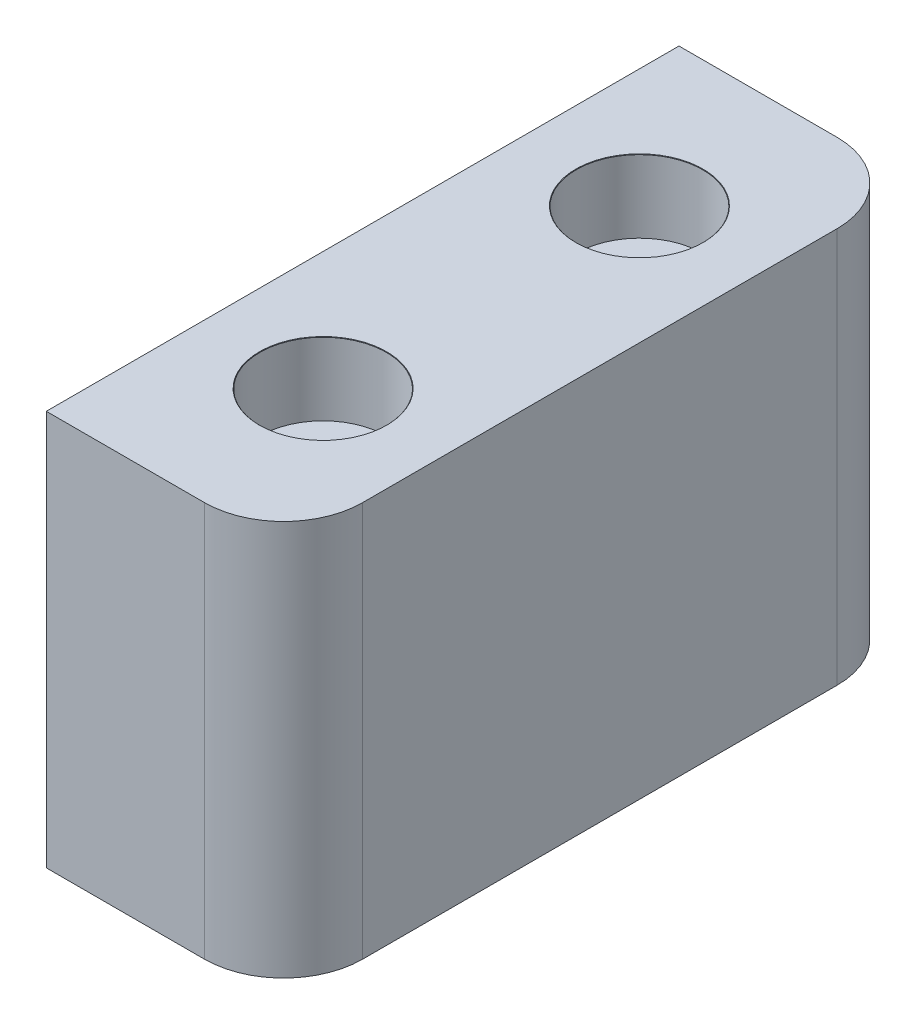
from build123d import *

# Parameters (mm, degrees)
SKETCH1_W                                 = 15
SKETCH1_H                                 = 40
BOSS_EXTRUDE1_DEPTH                       = 25
FILLET1_R                                 = 5
HOLE_WIZARD_SOCKET_HEAD_CAP_SCREW_2_COUNT = 2
HOLE_WIZARD_SOCKET_HEAD_CAP_SCREW_2_PITCH = 20


with BuildPart() as part:
    # Sketch1 → Boss-Extrude1 (new body)
    with BuildSketch(Plane(origin=(0, 0, 0), x_dir=(1, 0, 0), z_dir=(0, 1, 0))):
        Rectangle(SKETCH1_W, SKETCH1_H)
    extrude(amount=BOSS_EXTRUDE1_DEPTH)

    # Fillet1
    fillet1_edges = [part.edges().sort_by_distance(p)[0] for p in [
        (7.5, 12.5, 20),
        (7.5, 12.5, -20),
    ]]
    fillet(fillet1_edges, radius=FILLET1_R)

    # Sketch3 → Hole wizard: socket head cap screw, type 1 (revolve, cut)
    with BuildSketch(Plane(origin=(0, 25, -10), x_dir=(0, 0, 1), z_dir=(1, 0, 0))):
        Polygon((0, 0), (0, 25), (2.25, 25), (2.25, 4.6), (4, 4.6), (4, 0.025), (4.025, 0), align=None)
    hole_wizard_socket_head_cap_screw_type = revolve(axis=Axis((0, 31.35, -10), (0, -1, 0)), mode=Mode.SUBTRACT)

    # Hole wizard_ socket head cap screw_  2: Hole wizard: socket head cap screw, type 1 ×2
    with Locations(*[(0, 0, i * HOLE_WIZARD_SOCKET_HEAD_CAP_SCREW_2_PITCH) for i in range(1, HOLE_WIZARD_SOCKET_HEAD_CAP_SCREW_2_COUNT)]):
        add(hole_wizard_socket_head_cap_screw_type, mode=Mode.SUBTRACT)


solid = part.part
